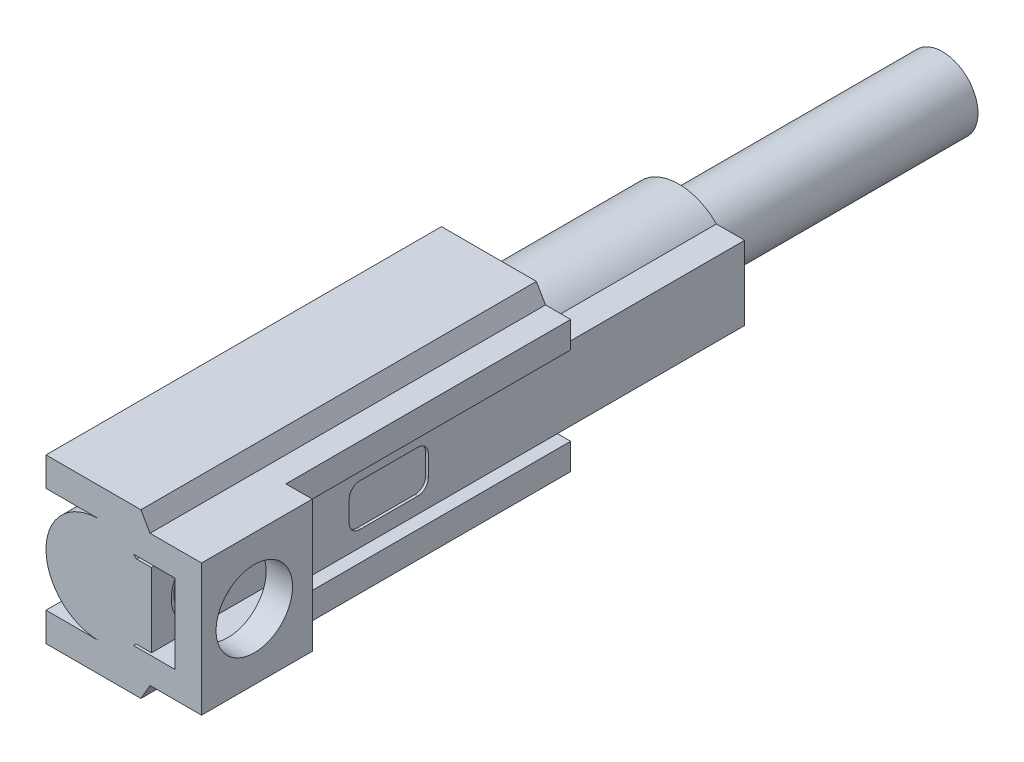
from build123d import *

# Parameters (mm, degrees)
EXTRUDE_1_DEPTH          = 15
SKETCH_2_W               = 1
SKETCH_2_H               = 5
CUT_EXTRUDE_1_DEPTH      = 10.8
SKETCH_3_R               = 1.45
CUT_EXTRUDE_2_DEPTH      = 1
EXTRUDE_2_DEPTH          = 22
CUT_EXTRUDE_3_DEPTH      = 1.4
CUT_EXTRUDE_3_DEPTH_BACK = 1.4
SKETCH_5_W               = 0.5
SKETCH_5_H               = 5
SKETCH_6_R               = 1.25
SKETCH_6_R_2             = 1.05
CUT_EXTRUDE_4_DEPTH      = 0.1
CUT_EXTRUDE_5_DEPTH      = 0.1
CUT_EXTRUDE_6_DEPTH      = 0.1
SKETCH_9_R               = 1.35
EXTRUDE_3_DEPTH          = 10


with BuildPart() as part:
    # 草图1 → 凸台-拉伸1 (new body)
    with BuildSketch(Plane.XY):
        with BuildLine():
            Line((-2, -3.1), (1.6, -3.1))
            Line((1.6, -3.1), (1.946410162, -2.5))
            Line((1.946410162, -2.5), (3.9, -2.5))
            Line((3.9, -2.5), (3.9, 2.5))
            Line((3.9, 2.5), (1.946410162, 2.5))
            Line((1.946410162, 2.5), (1.6, 3.1))
            Line((1.6, 3.1), (-2, 3.1))
            Line((-2, 3.1), (-2, 2))
            Line((-2, 2), (0, 2))
            ThreePointArc((0, 2), (0.707106781, 1.870828693), (1.322875656, 1.5))
            Line((1.322875656, 1.5), (2.9, 1.5))
            Line((2.9, 1.5), (2.9, -1.5))
            Line((2.9, -1.5), (1.322875656, -1.5))
            ThreePointArc((1.322875656, -1.5), (0.707106781, -1.870828693), (0, -2))
            Line((0, -2), (-2, -2))
            Line((-2, -2), (-2, -3.1))
        make_face()
    extrude(amount=-EXTRUDE_1_DEPTH)

    # 草图2 → 切除-拉伸1 (cut)
    with BuildSketch(Plane.XY.offset(-4.2)):
        with Locations((3.4, 0)):
            Rectangle(SKETCH_2_W, SKETCH_2_H)
    extrude(amount=-CUT_EXTRUDE_1_DEPTH, mode=Mode.SUBTRACT)

    # 草图3 → 切除-拉伸2 (cut)
    with BuildSketch(Plane(origin=(3.9, 0, 0), x_dir=(0, 0, -1), z_dir=(1, 0, 0))):
        with Locations((2, 0)):
            Circle(SKETCH_3_R)
    extrude(amount=-CUT_EXTRUDE_2_DEPTH, mode=Mode.SUBTRACT)

    # 草图4 → 凸台-拉伸2 (add)
    with BuildSketch(Plane.XY):
        with BuildLine():
            Line((1.428285686, -1.4), (2.5, -1.4))
            Line((2.5, -1.4), (2.5, 1.4))
            Line((2.5, 1.4), (1.428285686, 1.4))
            ThreePointArc((1.428285686, 1.4), (-2, 0), (1.428285686, -1.4))
        make_face()
    extrude(amount=-EXTRUDE_2_DEPTH)

    # 草图5 → 切除-拉伸3 (cut, two sides: drawn at the far end of the back side and taken through both)
    with BuildSketch(Plane(origin=(0, 0, 0), x_dir=(1, 0, 0), z_dir=(0, 1, 0)).offset(-CUT_EXTRUDE_3_DEPTH_BACK)):
        with Locations((2.25, 2.5)):
            Rectangle(SKETCH_5_W, SKETCH_5_H)
    extrude(amount=CUT_EXTRUDE_3_DEPTH + CUT_EXTRUDE_3_DEPTH_BACK, mode=Mode.SUBTRACT)

    # 草图6 → 切除-拉伸4 (cut)
    with BuildSketch(Plane(origin=(2, 0, 0), x_dir=(0, 0, -1), z_dir=(1, 0, 0))):
        with Locations((2, 0)):
            Circle(SKETCH_6_R)
        with Locations((2, 0)):
            Circle(SKETCH_6_R_2, mode=Mode.SUBTRACT)
    extrude(amount=-CUT_EXTRUDE_4_DEPTH, mode=Mode.SUBTRACT)

    # 草图7 → 切除-拉伸5 (cut)
    with BuildSketch(Plane(origin=(2, 0, 0), x_dir=(0, 0, -1), z_dir=(1, 0, 0))):
        with BuildLine():
            Line((0.966284129, 0.609451802), (2.609451802, -1.033715871))
            ThreePointArc((2.609451802, -1.033715871), (2.848528137, -0.848528137), (3.033715871, -0.609451802))
            Line((3.033715871, -0.609451802), (1.390548198, 1.033715871))
            ThreePointArc((1.390548198, 1.033715871), (1.151471863, 0.848528137), (0.966284129, 0.609451802))
        make_face()
    extrude(amount=-CUT_EXTRUDE_5_DEPTH, mode=Mode.SUBTRACT)

    # 草图8 → 切除-拉伸6 (cut)
    with BuildSketch(Plane(origin=(2.5, 0, 0), x_dir=(0, 0, -1), z_dir=(1, 0, 0))):
        with BuildLine():
            Line((7.4, -0.8), (9.6, -0.8))
            ThreePointArc((9.6, -0.8), (9.882842712, -0.682842712), (10, -0.4))
            Line((10, -0.4), (10, 0.4))
            ThreePointArc((10, 0.4), (9.882842712, 0.682842712), (9.6, 0.8))
            Line((9.6, 0.8), (7.4, 0.8))
            ThreePointArc((7.4, 0.8), (7.117157288, 0.682842712), (7, 0.4))
            Line((7, 0.4), (7, -0.4))
            ThreePointArc((7, -0.4), (7.117157288, -0.682842712), (7.4, -0.8))
        make_face()
    extrude(amount=-CUT_EXTRUDE_6_DEPTH, mode=Mode.SUBTRACT)

    # 草图9 → 凸台-拉伸3 (add)
    with BuildSketch(Plane.XY.offset(-22)):
        Circle(SKETCH_9_R)
    extrude(amount=-EXTRUDE_3_DEPTH)


solid = part.part
